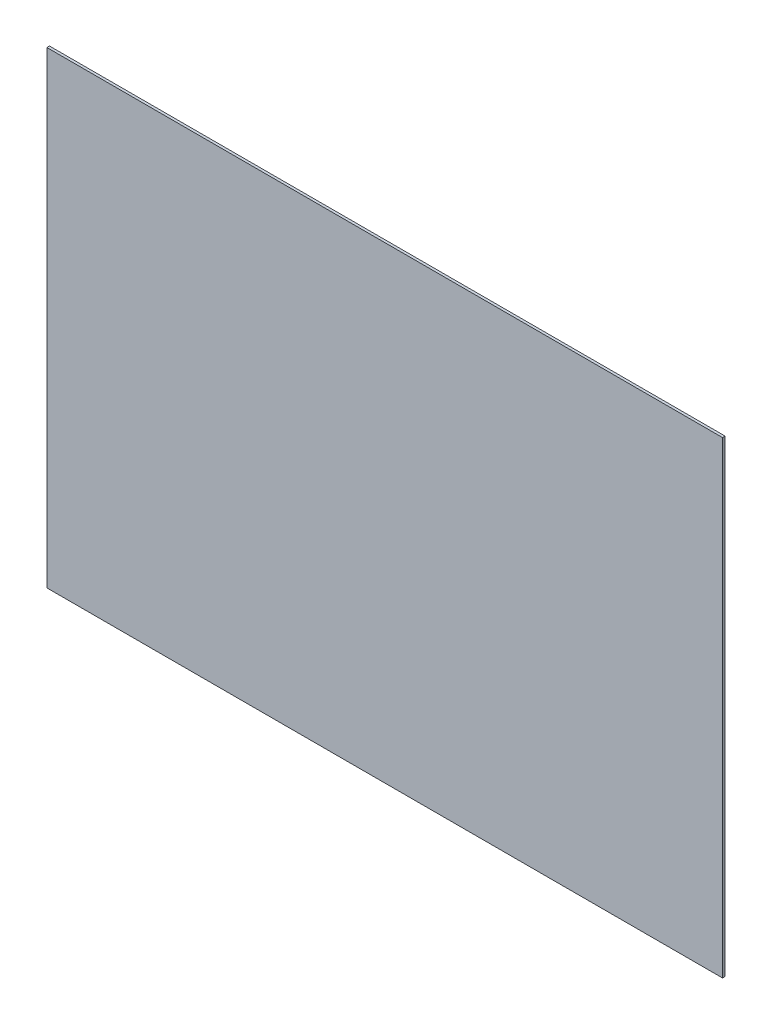
from build123d import *

# Parameters (mm, degrees)
SKETCH_1_W      = 1048
SKETCH_1_H      = 726
EXTRUDE_1_DEPTH = 4


with BuildPart() as part:
    # 草图1 → 凸台-拉伸1 (new body)
    with BuildSketch(Plane.XY):
        Rectangle(SKETCH_1_W, SKETCH_1_H)
    extrude(amount=EXTRUDE_1_DEPTH)


solid = part.part
